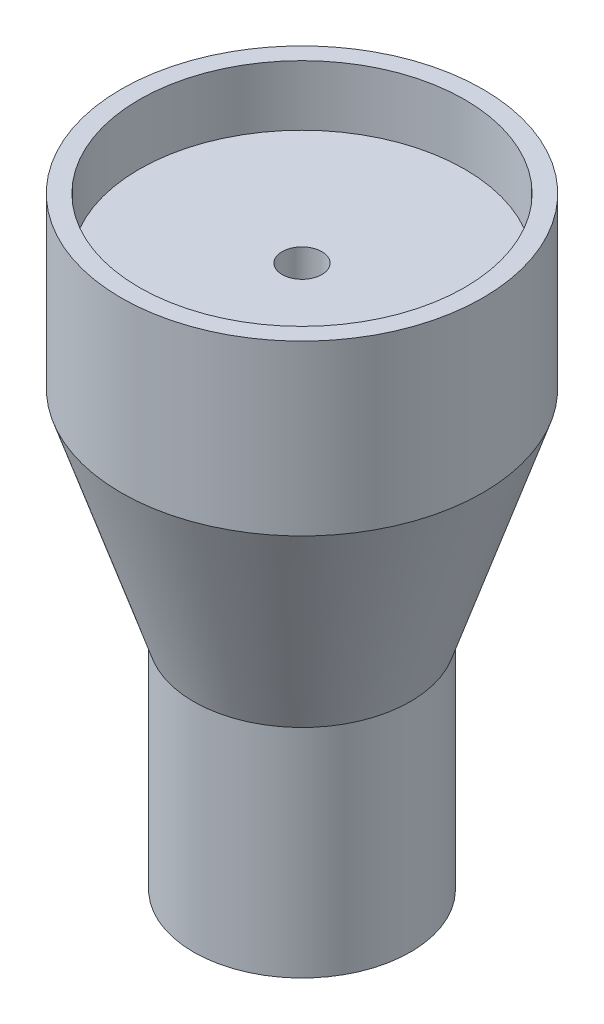
from build123d import *

# Parameters (mm, degrees)
M10X1_0_TAPPED_HOLE1_D     = 9
M10X1_0_TAPPED_HOLE1_DEPTH = 28
M10X1_0_TAPPED_HOLE1_TIP   = 2.703872786
M4_TAPPED_HOLE1_D          = 3.3
M4_TAPPED_HOLE1_DEPTH      = 10.1
M4_TAPPED_HOLE1_TIP        = 0.991420021


with BuildPart() as part:
    # Sketch1 → Revolve1 (revolve)
    with BuildSketch(Plane.XY, mode=Mode.PRIVATE) as revolve1_sk:
        Polygon((0, 0), (-9, 0), (-9, 18), (-15, 36), (-15, 50), (-13.5, 50), (-13.5, 45), (0, 45), align=None)
    revolve(revolve1_sk.sketch.rotate(Axis((0, 0, 0), (0, -1, 0)), 270), axis=Axis((0, 0, 0), (0, -1, 0)))

    # M10x1.0 Tapped Hole1
    with Locations(Plane(origin=(0, 0, 0), x_dir=(-1, 0, 0), z_dir=(0, -1, 0))):
        with Locations((0, 0)):
            Hole(M10X1_0_TAPPED_HOLE1_D / 2, depth=M10X1_0_TAPPED_HOLE1_DEPTH)
            with Locations((0, 0, -(M10X1_0_TAPPED_HOLE1_DEPTH + M10X1_0_TAPPED_HOLE1_TIP / 2))):  # 118° drill point
                Cone(0, M10X1_0_TAPPED_HOLE1_D / 2, M10X1_0_TAPPED_HOLE1_TIP, mode=Mode.SUBTRACT)

    # M4 Tapped Hole1
    with Locations(Plane(origin=(0, 45, 0), x_dir=(1, 0, 0), z_dir=(0, 1, 0))):
        with Locations((0, 0)):
            Hole(M4_TAPPED_HOLE1_D / 2, depth=M4_TAPPED_HOLE1_DEPTH)
            with Locations((0, 0, -(M4_TAPPED_HOLE1_DEPTH + M4_TAPPED_HOLE1_TIP / 2))):  # 118° drill point
                Cone(0, M4_TAPPED_HOLE1_D / 2, M4_TAPPED_HOLE1_TIP, mode=Mode.SUBTRACT)


solid = part.part
